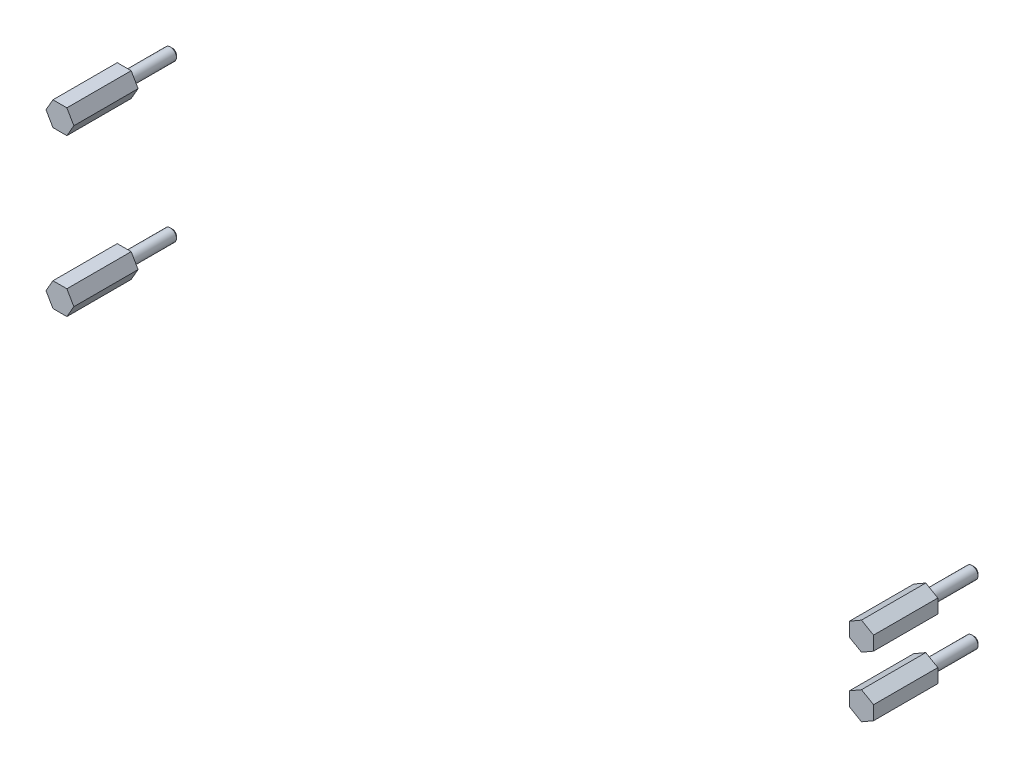
from build123d import *

# Parameters (mm, degrees)
BOSS_EXTRUDE1_DEPTH   = 16
BOSS_EXTRUDE1_2_DEPTH = 16
BOSS_EXTRUDE1_3_DEPTH = 16
BOSS_EXTRUDE1_4_DEPTH = 16
SKETCH_1_4_2_R        = 1.5
BOSS_EXTRUDE2_DEPTH   = 12
CHAMFER1_SIZE         = 0.5
CHAMFER2_SIZE         = 0.5
CHAMFER3_SIZE         = 0.5
CHAMFER4_SIZE         = 0.5


with BuildPart() as part:
    # Sketch 1_4 → Boss-Extrude1 (new body)
    with BuildSketch(Plane.XY):
        Polygon((117, -4.035898385), (114, -5.767949192), (114, -9.232050808), (117, -10.964101615), (120, -9.232050808), (120, -5.767949192), align=None)
    extrude(amount=BOSS_EXTRUDE1_DEPTH)



with BuildPart() as body_2:
    # Sketch 1_4 → Boss-Extrude1 2 (new body)
    with BuildSketch(Plane.XY):
        Polygon((120, 5.767949192), (117, 4.035898385), (114, 5.767949192), (114, 9.232050808), (117, 10.964101615), (120, 9.232050808), align=None)
    extrude(amount=BOSS_EXTRUDE1_2_DEPTH)


with BuildPart() as body_3:
    # Sketch 1_4 → Boss-Extrude1 3 (new body)
    with BuildSketch(Plane.XY):
        Polygon((-79.035898385, -19.5), (-80.767949192, -16.5), (-84.232050808, -16.5), (-85.964101615, -19.5), (-84.232050808, -22.5), (-80.767949192, -22.5), align=None)
    extrude(amount=BOSS_EXTRUDE1_3_DEPTH)


with BuildPart() as body_4:
    # Sketch 1_4 → Boss-Extrude1 4 (new body)
    with BuildSketch(Plane.XY):
        Polygon((-80.767949192, 22.5), (-79.035898385, 19.5), (-80.767949192, 16.5), (-84.232050808, 16.5), (-85.964101615, 19.5), (-84.232050808, 22.5), align=None)
    extrude(amount=BOSS_EXTRUDE1_4_DEPTH)


with BuildPart() as part_1:
    add(part.part)

    add(body_2.part)  # Boss-Extrude2 merges body 2

    add(body_3.part)  # Boss-Extrude2 merges body 3

    add(body_4.part)  # Boss-Extrude2 merges body 4
    # Sketch 1_4 2 → Boss-Extrude2 (add)
    with BuildSketch(Plane.XY):
        with Locations((-82.5, 19.5)):
            Circle(SKETCH_1_4_2_R)
        with Locations((-82.5, -19.5)):
            Circle(SKETCH_1_4_2_R)
        with Locations((117, 7.5)):
            Circle(SKETCH_1_4_2_R)
        with Locations((117, -7.5)):
            Circle(SKETCH_1_4_2_R)
    extrude(amount=-BOSS_EXTRUDE2_DEPTH)

    # Chamfer1
    chamfer1_edges = [part_1.edges().sort_by_distance(p)[0] for p in [
        (-84, 19.5, -12),
    ]]
    chamfer(chamfer1_edges, length=CHAMFER1_SIZE)

    # Chamfer2
    chamfer2_edges = [part_1.edges().sort_by_distance(p)[0] for p in [
        (-84, -19.5, -12),
    ]]
    chamfer(chamfer2_edges, length=CHAMFER2_SIZE)

    # Chamfer3
    chamfer3_edges = [part_1.edges().sort_by_distance(p)[0] for p in [
        (115.5, -7.5, -12),
    ]]
    chamfer(chamfer3_edges, length=CHAMFER3_SIZE)

    # Chamfer4
    chamfer4_edges = [part_1.edges().sort_by_distance(p)[0] for p in [
        (115.5, 7.5, -12),
    ]]
    chamfer(chamfer4_edges, length=CHAMFER4_SIZE)


solid = part_1.part
